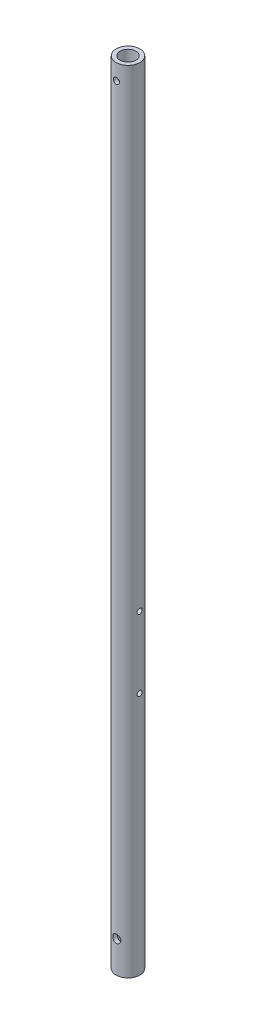
from build123d import *

# Parameters (mm, degrees)
SKETCH_1_R               = 6
SKETCH_1_R_2             = 4
EXTRUDE_1_DEPTH          = 400
CUT_EXTRUDE_1_DEPTH      = 401.089989877
CUT_EXTRUDE_1_DEPTH_BACK = 401.089989877
SKETCH_2_R               = 2.05
SKETCH_2_R_2             = 1.55
CUT_EXTRUDE_2_DEPTH      = 401.089989981
CUT_EXTRUDE_2_DEPTH_BACK = 401.089989981
SKETCH_3_R               = 1.3


with BuildPart() as part:
    # 草图1 → 凸台-拉伸1 (new body)
    with BuildSketch(Plane(origin=(0, 0, 0), x_dir=(1, 0, 0), z_dir=(0, 1, 0))):
        with Locations(Location((0, 0, 0), (0, 0, 270))):
            Circle(SKETCH_1_R)
        with Locations(Location((0, 0, 0), (0, 0, 270))):
            Circle(SKETCH_1_R_2, mode=Mode.SUBTRACT)
    extrude(amount=EXTRUDE_1_DEPTH)

    # 草图2 → 切除-拉伸1 (cut, two sides: drawn at the far end of the back side and taken through both)
    with BuildSketch(Plane.XY.offset(-CUT_EXTRUDE_1_DEPTH_BACK)):
        with Locations((0, 16)):
            Circle(SKETCH_2_R)
        with Locations((0, 392)):
            Circle(SKETCH_2_R_2)
    extrude(amount=CUT_EXTRUDE_1_DEPTH + CUT_EXTRUDE_1_DEPTH_BACK, mode=Mode.SUBTRACT)

    # 草图3 → 切除-拉伸2 (cut, two sides: drawn at the far end of the back side and taken through both)
    with BuildSketch(Plane(origin=(0, 0, 0), x_dir=(0, 0, -1), z_dir=(1, 0, 0)).offset(-CUT_EXTRUDE_2_DEPTH_BACK)):
        with Locations((0, 159.5)):
            Circle(SKETCH_3_R)
        with Locations((0, 123.5)):
            Circle(SKETCH_3_R)
    extrude(amount=CUT_EXTRUDE_2_DEPTH + CUT_EXTRUDE_2_DEPTH_BACK, mode=Mode.SUBTRACT)


solid = part.part
